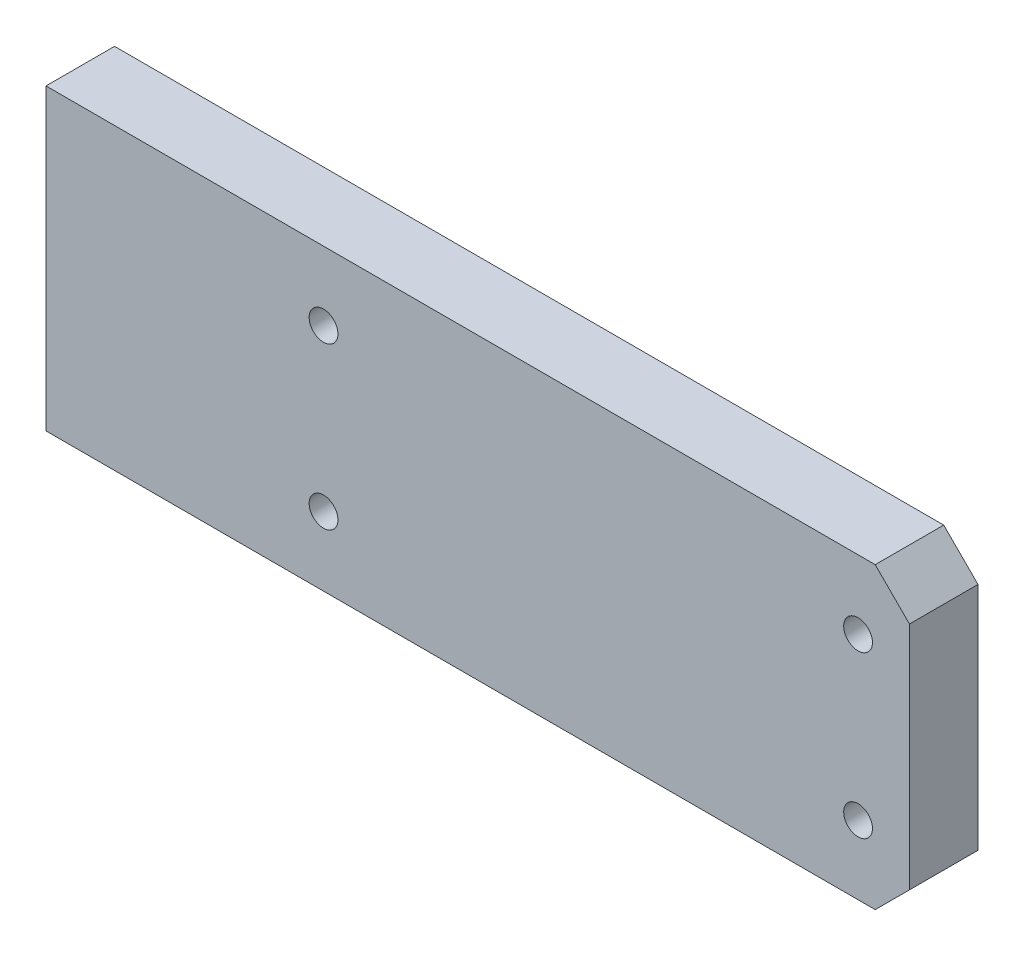
SolidWorks part; units mm, degrees
ref_plane "前视基准面" through (0, 0, 0) normal (0, 0, 1) x (1, 0, 0)
ref_plane "上视基准面" through (0, 0, 0) normal (0, 1, 0) x (1, 0, 0)
ref_plane "右视基准面" through (0, 0, 0) normal (1, 0, 0) x (0, 0, -1)
sketch "草图1" plane through (0, 0, 0) normal (0, 1, 0) x (1, 0, 0)
  line L1 (0, 0) -> (126, 0)
  line L2 (0, 0) -> (0, 10)
  line L3 (0, 10) -> (126, 10)
  line L4 (126, 0) -> (126, 10)
  dimension "D1" = 10
  dimension "D2" = 126
extrude "凸台-拉伸1" add sketch "草图1" along normal blind 43.6
chamfer "倒角1" distance 5 angle 45 2 edges at (126, 0, -5) (126, 43.6, -5)
sketch "草图4" plane through (0, 0, 0) normal (-1, 0, 0) x (0, 0, 1)
  point P0 (-5, 36.8)
  point P3 (-5, 21.7835)
  point P6 (-5, 6.8)
hole_wizard "M4 螺纹孔1" positions "草图4" profile "草图3" tap size "M4" standard "GB"
sketch "草图3" plane through (0, 36.8, -5) normal (0, 1, 0) x (0, 0, 1)
  line L0 (0, 0) -> (0, 11.0914)
  line L1 (0, 11.0914) -> (1.65, 10.1)
  line L2 (1.65, 10.1) -> (1.65, 0)
  line L5 (1.65, 0) -> (0, 0)
  line L10 (0, 11.0914) -> (-1.65, 10.1) construction
  line L11 (0, -6.35) -> (0, 107.95) construction
  dimension "螺纹孔钻头直径" = 3.3
  dimension "螺纹孔钻头深度" = 10.1
  dimension "导头角度" = 118
cosmetic thread "孔螺纹线1" parameters "D1"=8, "D2"=4
cosmetic thread "孔螺纹线2" parameters "D1"=8, "D2"=4
cosmetic thread "孔螺纹线3" parameters "D1"=8, "D2"=4
sketch "草图7" plane through (0, 0, -10) normal (0, 0, -1) x (-1, 0, 0)
  line L7 (-126, 21.8) -> (-62.8352, 21.8) construction
  line L8 (-126, 38.6) -> (-126, 5) construction
  point P0 (-40.5, 33.55)
  point P2 (-40.5, 10.05)
  point P4 (-118.5, 33.55)
  point P6 (-118.5, 10.05)
  dimension "D1" = 23.5
  dimension "D2" = 23.5
  dimension "D3" = 78
  dimension "D4" = 7.5
hole_wizard "M5 螺纹孔1" positions "草图7" profile "草图6" tap size "M5" standard "GB" end condition through all
sketch "草图6" plane through (40.5, 33.55, -10) normal (1, 0, 0) x (0, 1, 0)
  line L0 (0, 0) -> (0, 10)
  line L1 (0, 10) -> (2.1, 10)
  line L2 (2.1, 10) -> (2.1, 0)
  line L5 (2.1, 0) -> (0, 0)
  line L11 (0, -6.35) -> (0, 107.95) construction
  dimension "通孔螺纹孔钻头直径" = 4.2
  dimension "通孔螺纹孔钻头深度" = 10
cosmetic thread "孔螺纹线4" parameters "D2"=5
cosmetic thread "孔螺纹线5" parameters "D2"=5
cosmetic thread "孔螺纹线6" parameters "D2"=5
cosmetic thread "孔螺纹线7" parameters "D2"=5
